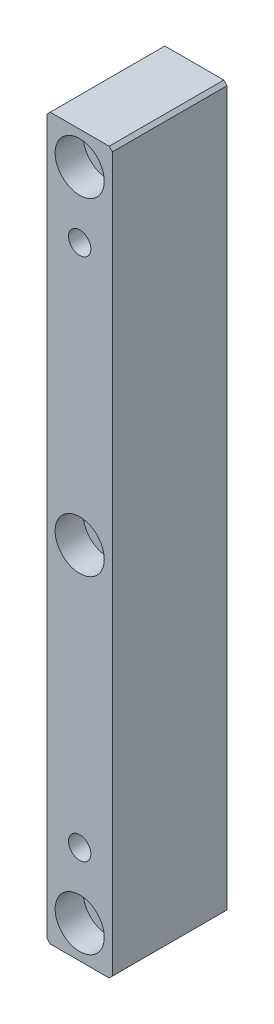
from build123d import *

# Parameters (mm, degrees)
SKETCH_1_W                   = 20
SKETCH_1_H                   = 220
EXTRUDE_1_DEPTH              = 17.5
HOLE_WIZARD_M8_1_D           = 9
HOLE_WIZARD_M8_1_CBORE_D     = 15
HOLE_WIZARD_M8_1_CBORE_DEPTH = 8.6
HOLE_WIZARD_M8_1_2_D         = 6.8
HOLE_WIZARD_M8_1_2_DEPTH     = 19.75
HOLE_WIZARD_M8_1_2_TIP       = 2.042926105
CHAMFER_1_SIZE               = 1


with BuildPart() as part:
    # 草图1 → 凸台-拉伸1 (new, symmetric)
    with BuildSketch(Plane.XY):
        Rectangle(SKETCH_1_W, SKETCH_1_H)
    extrude(amount=EXTRUDE_1_DEPTH, both=True)

    # Hole Wizard M8 _1 (through all)
    with Locations(Plane.XY.offset(17.5)):
        with Locations((0, 100), (0, 0), (0, -100)):
            CounterBoreHole(HOLE_WIZARD_M8_1_D / 2, HOLE_WIZARD_M8_1_CBORE_D / 2, HOLE_WIZARD_M8_1_CBORE_DEPTH)

    # Hole Wizard M8 _1 2
    with Locations(Plane.XY.offset(17.5)):
        with Locations((0, 80), (0, -80)):
            Hole(HOLE_WIZARD_M8_1_2_D / 2, depth=HOLE_WIZARD_M8_1_2_DEPTH)
            with Locations((0, 0, -(HOLE_WIZARD_M8_1_2_DEPTH + HOLE_WIZARD_M8_1_2_TIP / 2))):  # 118° drill point
                Cone(0, HOLE_WIZARD_M8_1_2_D / 2, HOLE_WIZARD_M8_1_2_TIP, mode=Mode.SUBTRACT)

    # 倒角1
    chamfer_1_edges = [part.edges().sort_by_distance(p)[0] for p in [
        (10, -110, 0),
        (-10, -110, 0),
        (-10, 110, 0),
        (10, 110, 0),
    ]]
    chamfer(chamfer_1_edges, length=CHAMFER_1_SIZE)


solid = part.part
